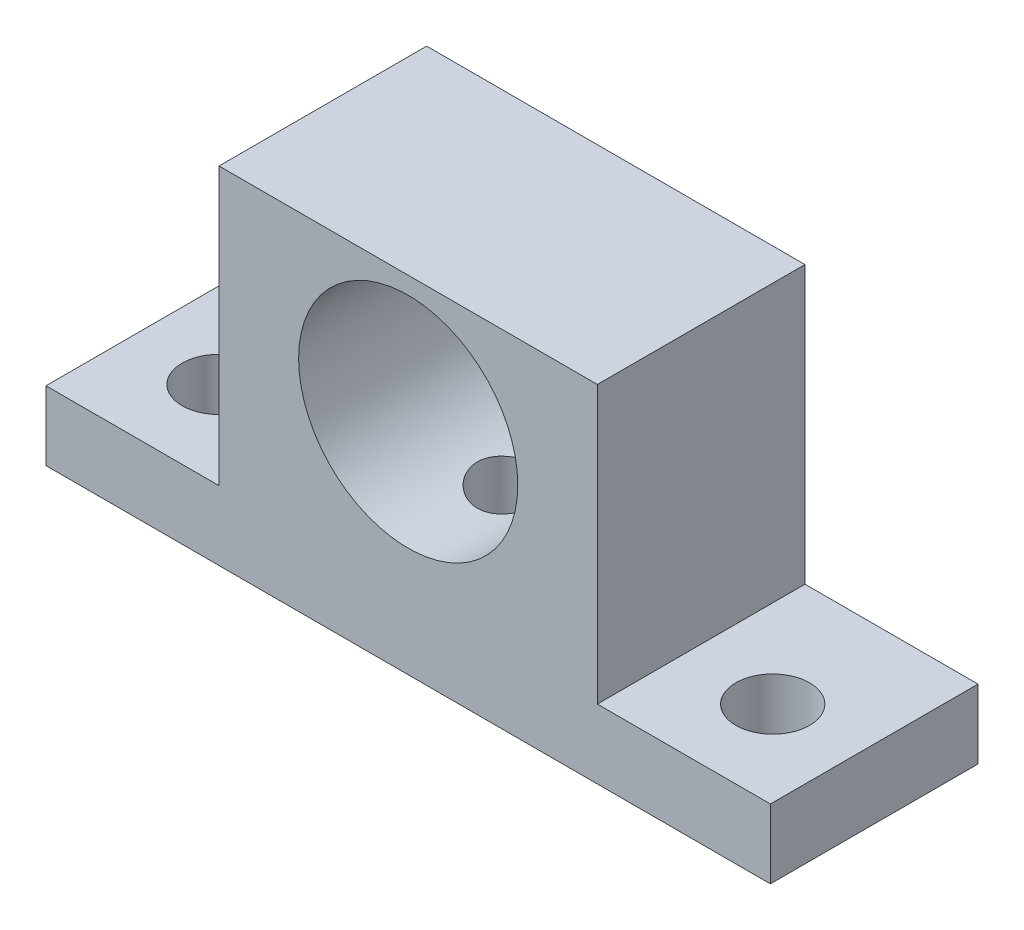
from build123d import *

# Parameters (mm, degrees)
SKETCH1_W           = 40.4
SKETCH1_H           = 20
BOSS_EXTRUDE1_DEPTH = 15
SKETCH2_R           = 4.75
CUT_EXTRUDE1_DEPTH  = 36
SKETCH3_R           = 1.6
CUT_EXTRUDE2_DEPTH  = 36
SKETCH4_W           = 40.4
SKETCH4_H           = 8.8
CUT_EXTRUDE3_DEPTH  = 36
SKETCH5_W           = 40.4
SKETCH5_H           = 2.2
CUT_EXTRUDE4_DEPTH  = 36
SKETCH8_W           = 12
SKETCH8_H           = 9
CUT_EXTRUDE6_DEPTH  = 12
SKETCH10_W          = 4.5
SKETCH10_H          = 9
CUT_EXTRUDE7_DEPTH  = 12
SKETCH11_R          = 1.5
CUT_EXTRUDE8_DEPTH  = 10


with BuildPart() as part:
    # Sketch1 → Boss-Extrude1 (new body)
    with BuildSketch(Plane(origin=(0, 0, 0), x_dir=(1, 0, 0), z_dir=(0, 1, 0))):
        with Locations((20.2, -10)):
            Rectangle(SKETCH1_W, SKETCH1_H)
    extrude(amount=BOSS_EXTRUDE1_DEPTH)

    # Sketch2 → Cut-Extrude1 (cut)
    with BuildSketch(Plane.XY.offset(20)):
        with Locations((20.2, 9.5)):
            Circle(SKETCH2_R)
    extrude(amount=-CUT_EXTRUDE1_DEPTH, mode=Mode.SUBTRACT)

    # Sketch3 → Cut-Extrude2 (cut)
    with BuildSketch(Plane(origin=(0, 15, 0), x_dir=(1, 0, 0), z_dir=(0, 1, 0))):
        with Locations(Location((8.2, -14, 0), (0, 0, 270))):
            Circle(SKETCH3_R)
        with Locations(Location((32.2, -14, 0), (0, 0, 270))):
            Circle(SKETCH3_R)
    extrude(amount=-CUT_EXTRUDE2_DEPTH, mode=Mode.SUBTRACT)

    # Sketch4 → Cut-Extrude3 (cut)
    with BuildSketch(Plane(origin=(0, 15, 0), x_dir=(1, 0, 0), z_dir=(0, 1, 0))):
        with Locations((20.2, -4.4)):
            Rectangle(SKETCH4_W, SKETCH4_H)
    extrude(amount=-CUT_EXTRUDE3_DEPTH, mode=Mode.SUBTRACT)

    # Sketch5 → Cut-Extrude4 (cut)
    with BuildSketch(Plane(origin=(0, 15, 0), x_dir=(1, 0, 0), z_dir=(0, 1, 0))):
        with Locations((20.2, -18.9)):
            Rectangle(SKETCH5_W, SKETCH5_H)
    extrude(amount=-CUT_EXTRUDE4_DEPTH, mode=Mode.SUBTRACT)

    # Sketch8 → Cut-Extrude6 (cut)
    with BuildSketch(Plane(origin=(0, 15, 0), x_dir=(1, 0, 0), z_dir=(0, 1, 0))):
        with Locations((6, -13.3)):
            Rectangle(SKETCH8_W, SKETCH8_H)
        with Locations((34.4, -13.3)):
            Rectangle(SKETCH8_W, SKETCH8_H)
    extrude(amount=-CUT_EXTRUDE6_DEPTH, mode=Mode.SUBTRACT)

    # Sketch10 → Cut-Extrude7 (cut)
    with BuildSketch(Plane(origin=(0, 3, 0), x_dir=(1, 0, 0), z_dir=(0, 1, 0))):
        with Locations((2.25, -13.3)):
            Rectangle(SKETCH10_W, SKETCH10_H)
        with Locations((38.15, -13.3)):
            Rectangle(SKETCH10_W, SKETCH10_H)
    extrude(amount=-CUT_EXTRUDE7_DEPTH, mode=Mode.SUBTRACT)

    # Sketch11 → Cut-Extrude8 (cut)
    with BuildSketch(Plane.XZ):
        with Locations(Location((20.2, 13.3, 0), (0, 0, 270))):
            Circle(SKETCH11_R)
    extrude(amount=-CUT_EXTRUDE8_DEPTH, mode=Mode.SUBTRACT)


solid = part.part
